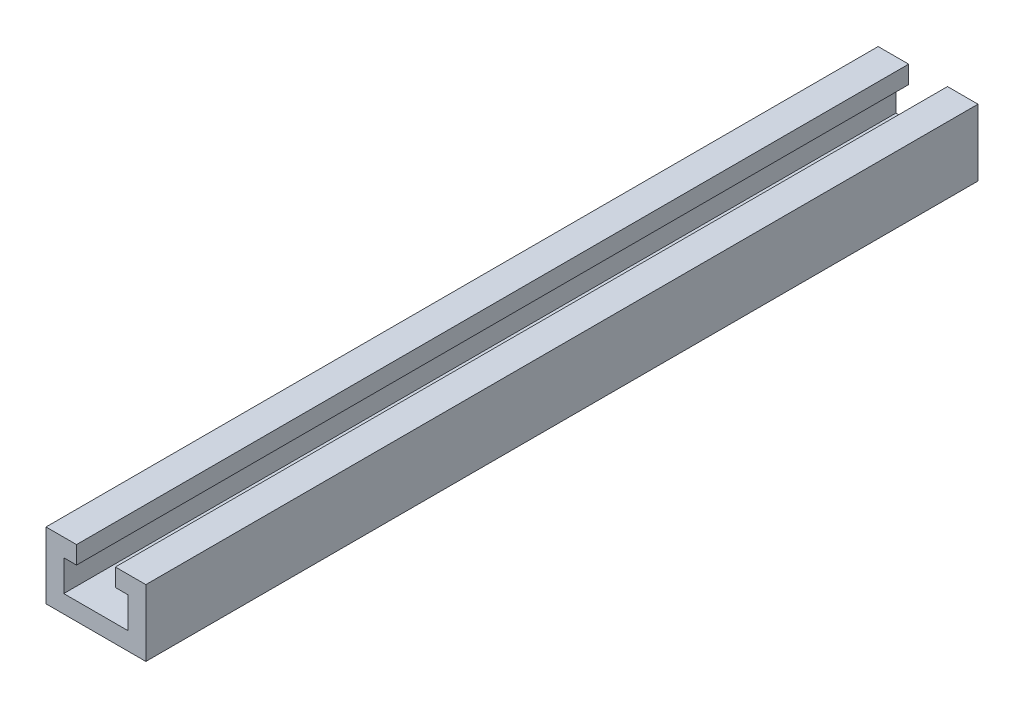
SolidWorks part; units mm, degrees
ref_plane "前视基准面" through (0, 0, 0) normal (0, 0, 1) x (1, 0, 0)
ref_plane "上视基准面" through (0, 0, 0) normal (0, 1, 0) x (1, 0, 0)
ref_plane "右视基准面" through (0, 0, 0) normal (1, 0, 0) x (0, 0, -1)
sketch "草图1" plane through (0, 0, 0) normal (0, 0, 1) x (1, 0, 0)
  line L0 (0, 0) -> (-4.5, 0)
  line L1 (-4.5, 0) -> (-4.5, 6)
  line L2 (-4.5, 6) -> (-1.75, 6)
  line L3 (-1.75, 6) -> (-1.75, 4.4)
  line L4 (-1.75, 4.4) -> (-2.9, 4.4)
  line L5 (-2.9, 4.4) -> (-2.9, 1.6)
  line L6 (-2.9, 1.6) -> (2.9, 1.6)
  line L7 (2.9, 1.6) -> (2.9, 4.4)
  line L8 (2.9, 4.4) -> (1.75, 4.4)
  line L9 (1.75, 4.4) -> (1.75, 6)
  line L10 (1.75, 6) -> (4.5, 6)
  line L11 (4.5, 6) -> (4.5, 0)
  line L12 (4.5, 0) -> (0, 0)
  dimension "D1" = 9
  dimension "D2" = 6
  dimension "D3" = 3.5
  dimension "D4" = 5.8
  dimension "D5" = 1.6
  dimension "D6" = 1.6
  dimension "D7" = 1.6
extrude "凸台-拉伸1" add sketch "草图1" along normal mid plane 75
